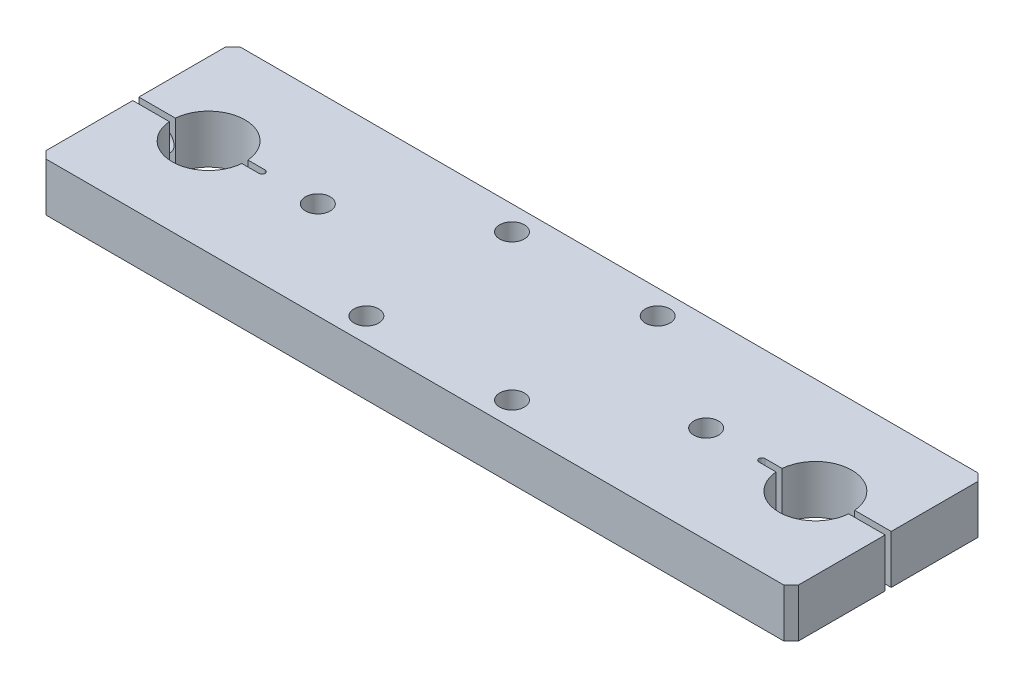
from build123d import *

# Parameters (mm, degrees)
SKETCH_1_W                  = 310
SKETCH_1_H                  = 80
EXTRUDE_1_DEPTH             = 10
SKETCH_2_R                  = 15
CUT_EXTRUDE_1_DEPTH         = 20
CHAMFER_1_SIZE              = 3
CUT_EXTRUDE_2_DEPTH         = 20
HOLE_WIZARD_2_D             = 9
HOLE_WIZARD_2_DEPTH         = 40
HOLE_WIZARD_2_CBORE_D       = 15
HOLE_WIZARD_2_CBORE_DEPTH   = 9
HOLE_WIZARD_2_TIP           = 2.703872786
HOLE_WIZARD_M8_1_D          = 6.8
HOLE_WIZARD_M8_1_DEPTH      = 19.75
HOLE_WIZARD_M8_1_TIP        = 2.042926105
HOLE_WIZARD_2_2_D           = 11
HOLE_WIZARD_2_2_DEPTH       = 19.75
HOLE_WIZARD_2_2_CBORE_D     = 18
HOLE_WIZARD_2_2_CBORE_DEPTH = 11
HOLE_WIZARD_2_2_TIP         = 3.304733405
HOLE_WIZARD_M12_1_D         = 10.2


with BuildPart() as part:
    # 草图1 → 凸台-拉伸1 (new, symmetric)
    with BuildSketch(Plane(origin=(0, 0, 0), x_dir=(1, 0, 0), z_dir=(0, 1, 0))):
        Rectangle(SKETCH_1_W, SKETCH_1_H)
    extrude(amount=EXTRUDE_1_DEPTH, both=True)

    # 草图2 → 切除-拉伸1 (cut)
    with BuildSketch(Plane(origin=(0, 10, 0), x_dir=(1, 0, 0), z_dir=(0, 1, 0))):
        with Locations(Location((125, 0, 0), (0, 0, 270))):
            Circle(SKETCH_2_R)
        with Locations(Location((-125, 0, 0), (0, 0, 90))):
            Circle(SKETCH_2_R)
    extrude(amount=-CUT_EXTRUDE_1_DEPTH, mode=Mode.SUBTRACT)

    # 倒角1
    chamfer_1_edges = [part.edges().sort_by_distance(p)[0] for p in [
        (155, 0, 40),
        (-155, 0, 40),
        (-155, 0, -40),
        (155, 0, -40),
    ]]
    chamfer(chamfer_1_edges, length=CHAMFER_1_SIZE)

    # 草图3 → 切除-拉伸2 (cut)
    with BuildSketch(Plane(origin=(0, 10, 0), x_dir=(1, 0, 0), z_dir=(0, 1, 0))):
        with BuildLine():
            Line((155, -1.25), (103, -1.25))
            ThreePointArc((103, -1.25), (101.75, 0), (103, 1.25))
            Line((103, 1.25), (155, 1.25))
            ThreePointArc((155, 1.25), (156.25, 0), (155, -1.25))
        make_face()
        with BuildLine():
            Line((-155, -1.25), (-103, -1.25))
            ThreePointArc((-103, -1.25), (-101.75, 0), (-103, 1.25))
            Line((-103, 1.25), (-155, 1.25))
            ThreePointArc((-155, 1.25), (-156.25, 0), (-155, -1.25))
        make_face()
    extrude(amount=-CUT_EXTRUDE_2_DEPTH, mode=Mode.SUBTRACT)

    # Hole Wizard 2
    with Locations(Plane(origin=(0, 0, -40), x_dir=(-1, 0, 0), z_dir=(0, 0, -1))):
        with Locations((-145, 0), (145, 0)):
            CounterBoreHole(HOLE_WIZARD_2_D / 2, HOLE_WIZARD_2_CBORE_D / 2, HOLE_WIZARD_2_CBORE_DEPTH, depth=HOLE_WIZARD_2_DEPTH)
            with Locations((0, 0, -(HOLE_WIZARD_2_DEPTH + HOLE_WIZARD_2_TIP / 2))):  # 118° drill point
                Cone(0, HOLE_WIZARD_2_D / 2, HOLE_WIZARD_2_TIP, mode=Mode.SUBTRACT)

    # M8 螺纹孔1
    with Locations(Plane(origin=(0, 0, 1.25), x_dir=(-1, 0, 0), z_dir=(0, 0, -1))):
        with Locations((-145, 0), (145, 0)):
            Hole(HOLE_WIZARD_M8_1_D / 2, depth=HOLE_WIZARD_M8_1_DEPTH)
            with Locations((0, 0, -(HOLE_WIZARD_M8_1_DEPTH + HOLE_WIZARD_M8_1_TIP / 2))):  # 118° drill point
                Cone(0, HOLE_WIZARD_M8_1_D / 2, HOLE_WIZARD_M8_1_TIP, mode=Mode.SUBTRACT)

    # Hole Wizard 2 2
    with Locations(Plane(origin=(0, -10, 0), x_dir=(-1, 0, 0), z_dir=(0, -1, 0))):
        with Locations((-30, 30), (30, 30), (30, -30), (-30, -30)):
            CounterBoreHole(HOLE_WIZARD_2_2_D / 2, HOLE_WIZARD_2_2_CBORE_D / 2, HOLE_WIZARD_2_2_CBORE_DEPTH, depth=HOLE_WIZARD_2_2_DEPTH)
            with Locations((0, 0, -(HOLE_WIZARD_2_2_DEPTH + HOLE_WIZARD_2_2_TIP / 2))):  # 118° drill point
                Cone(0, HOLE_WIZARD_2_2_D / 2, HOLE_WIZARD_2_2_TIP, mode=Mode.SUBTRACT)

    # M12 螺纹孔1 (through all)
    with Locations(Plane(origin=(0, 10, 0), x_dir=(1, 0, 0), z_dir=(0, 1, 0))):
        with Locations((80, 0), (-80, 0)):
            Hole(HOLE_WIZARD_M12_1_D / 2)


solid = part.part
